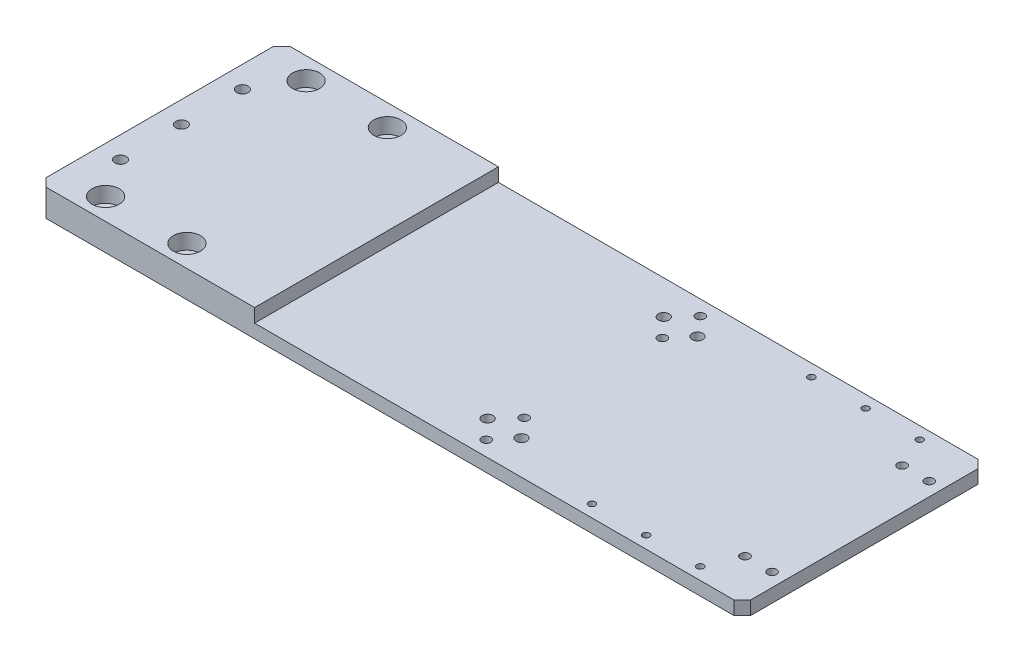
from build123d import *

# Parameters (mm, degrees)
SKETCH_1_W                = 260
SKETCH_1_H                = 90
EXTRUDE_1_DEPTH           = 10
CHAMFER_1_SIZE            = 3
HOLE_WIZARD_1_D           = 5.5
HOLE_WIZARD_1_DEPTH       = 10.1
HOLE_WIZARD_1_CBORE_D     = 10
HOLE_WIZARD_1_CBORE_DEPTH = 5.7
HOLE_WIZARD_1_TIP         = 1.652366702
HOLE_WIZARD_M5_1_D        = 4.2
HOLE_WIZARD_M5_1_DEPTH    = 12.4
HOLE_WIZARD_M5_1_TIP      = 1.2618073
SKETCH_8_W                = 180
SKETCH_8_H                = 90
CUT_EXTRUDE_1_DEPTH       = 5
HOLE_WIZARD_M3_1_D        = 2.5
HOLE_WIZARD_M3_1_DEPTH    = 7.5
HOLE_WIZARD_M3_1_TIP      = 0.751075774
HOLE_WIZARD_M4_1_D        = 3.3
HOLE_WIZARD_M4_1_DEPTH    = 20
HOLE_WIZARD_M4_1_TIP      = 0.991420021
HOLE_WIZARD_M4_2_D        = 3.3
HOLE_WIZARD_M4_2_DEPTH    = 20
HOLE_WIZARD_M4_2_TIP      = 0.991420021
MM_1_D                    = 4
MM_1_DEPTH                = 20
MM_1_TIP                  = 1.201721238


with BuildPart() as part:
    # 草图1 → 凸台-拉伸1 (new body)
    with BuildSketch(Plane(origin=(0, 0, 0), x_dir=(1, 0, 0), z_dir=(0, 1, 0))):
        Rectangle(SKETCH_1_W, SKETCH_1_H)
    extrude(amount=EXTRUDE_1_DEPTH)

    # 倒角1
    chamfer_1_edges = [part.edges().sort_by_distance(p)[0] for p in [
        (130, 5, 45),
        (-130, 5, 45),
        (-130, 5, -45),
        (130, 5, -45),
    ]]
    chamfer(chamfer_1_edges, length=CHAMFER_1_SIZE)

    # 打孔尺寸(%根据)内六角圆柱头螺钉的类型1
    with Locations(Plane(origin=(0, 10, 0), x_dir=(1, 0, 0), z_dir=(0, 1, 0))):
        with Locations((-83, 37), (-113, 37), (-83, -37), (-113, -37)):
            CounterBoreHole(HOLE_WIZARD_1_D / 2, HOLE_WIZARD_1_CBORE_D / 2, HOLE_WIZARD_1_CBORE_DEPTH, depth=HOLE_WIZARD_1_DEPTH)
            with Locations((0, 0, -(HOLE_WIZARD_1_DEPTH + HOLE_WIZARD_1_TIP / 2))):  # 118° drill point
                Cone(0, HOLE_WIZARD_1_D / 2, HOLE_WIZARD_1_TIP, mode=Mode.SUBTRACT)

    # M5 螺纹孔1
    with Locations(Plane(origin=(0, 10, 0), x_dir=(1, 0, 0), z_dir=(0, 1, 0))):
        with Locations((-122, 22.5), (-122, 0), (-122, -22.5)):
            Hole(HOLE_WIZARD_M5_1_D / 2, depth=HOLE_WIZARD_M5_1_DEPTH)
            with Locations((0, 0, -(HOLE_WIZARD_M5_1_DEPTH + HOLE_WIZARD_M5_1_TIP / 2))):  # 118° drill point
                Cone(0, HOLE_WIZARD_M5_1_D / 2, HOLE_WIZARD_M5_1_TIP, mode=Mode.SUBTRACT)

    # 草图8 → 切除-拉伸1 (cut)
    with BuildSketch(Plane(origin=(0, 10, 0), x_dir=(1, 0, 0), z_dir=(0, 1, 0))):
        with Locations((40, 0)):
            Rectangle(SKETCH_8_W, SKETCH_8_H)
    extrude(amount=-CUT_EXTRUDE_1_DEPTH, mode=Mode.SUBTRACT)

    # M3 螺纹孔1
    with Locations(Plane(origin=(0, 5, 0), x_dir=(1, 0, 0), z_dir=(0, 1, 0))):
        with Locations((110, -40.5), (90, -40.5), (70, -40.5), (110, 40.5), (90, 40.5), (70, 40.5)):
            Hole(HOLE_WIZARD_M3_1_D / 2, depth=HOLE_WIZARD_M3_1_DEPTH)
            with Locations((0, 0, -(HOLE_WIZARD_M3_1_DEPTH + HOLE_WIZARD_M3_1_TIP / 2))):  # 118° drill point
                Cone(0, HOLE_WIZARD_M3_1_D / 2, HOLE_WIZARD_M3_1_TIP, mode=Mode.SUBTRACT)

    # M4 螺纹孔1
    with Locations(Plane(origin=(0, 5, 0), x_dir=(1, 0, 0), z_dir=(0, 1, 0))):
        with Locations((115, -29), (125, -29), (115, 29), (125, 29)):
            Hole(HOLE_WIZARD_M4_1_D / 2, depth=HOLE_WIZARD_M4_1_DEPTH)
            with Locations((0, 0, -(HOLE_WIZARD_M4_1_DEPTH + HOLE_WIZARD_M4_1_TIP / 2))):  # 118° drill point
                Cone(0, HOLE_WIZARD_M4_1_D / 2, HOLE_WIZARD_M4_1_TIP, mode=Mode.SUBTRACT)

    # M4 螺纹孔2
    with Locations(Plane(origin=(0, 10, 0), x_dir=(1, 0, 0), z_dir=(0, 1, 0))):
        with Locations((30, -25.5), (30, -39.5), (30, 25.5), (30, 39.5)):
            Hole(HOLE_WIZARD_M4_2_D / 2, depth=HOLE_WIZARD_M4_2_DEPTH)
            with Locations((0, 0, -(HOLE_WIZARD_M4_2_DEPTH + HOLE_WIZARD_M4_2_TIP / 2))):  # 118° drill point
                Cone(0, HOLE_WIZARD_M4_2_D / 2, HOLE_WIZARD_M4_2_TIP, mode=Mode.SUBTRACT)

    # 大小mm 暗销孔1
    with Locations(Plane(origin=(0, 5, 0), x_dir=(1, 0, 0), z_dir=(0, 1, 0))):
        with Locations((23.5, -32.5), (36, -32.5), (23.5, 32.5), (36, 32.5)):
            Hole(MM_1_D / 2, depth=MM_1_DEPTH)
            with Locations((0, 0, -(MM_1_DEPTH + MM_1_TIP / 2))):  # 118° drill point
                Cone(0, MM_1_D / 2, MM_1_TIP, mode=Mode.SUBTRACT)


solid = part.part
